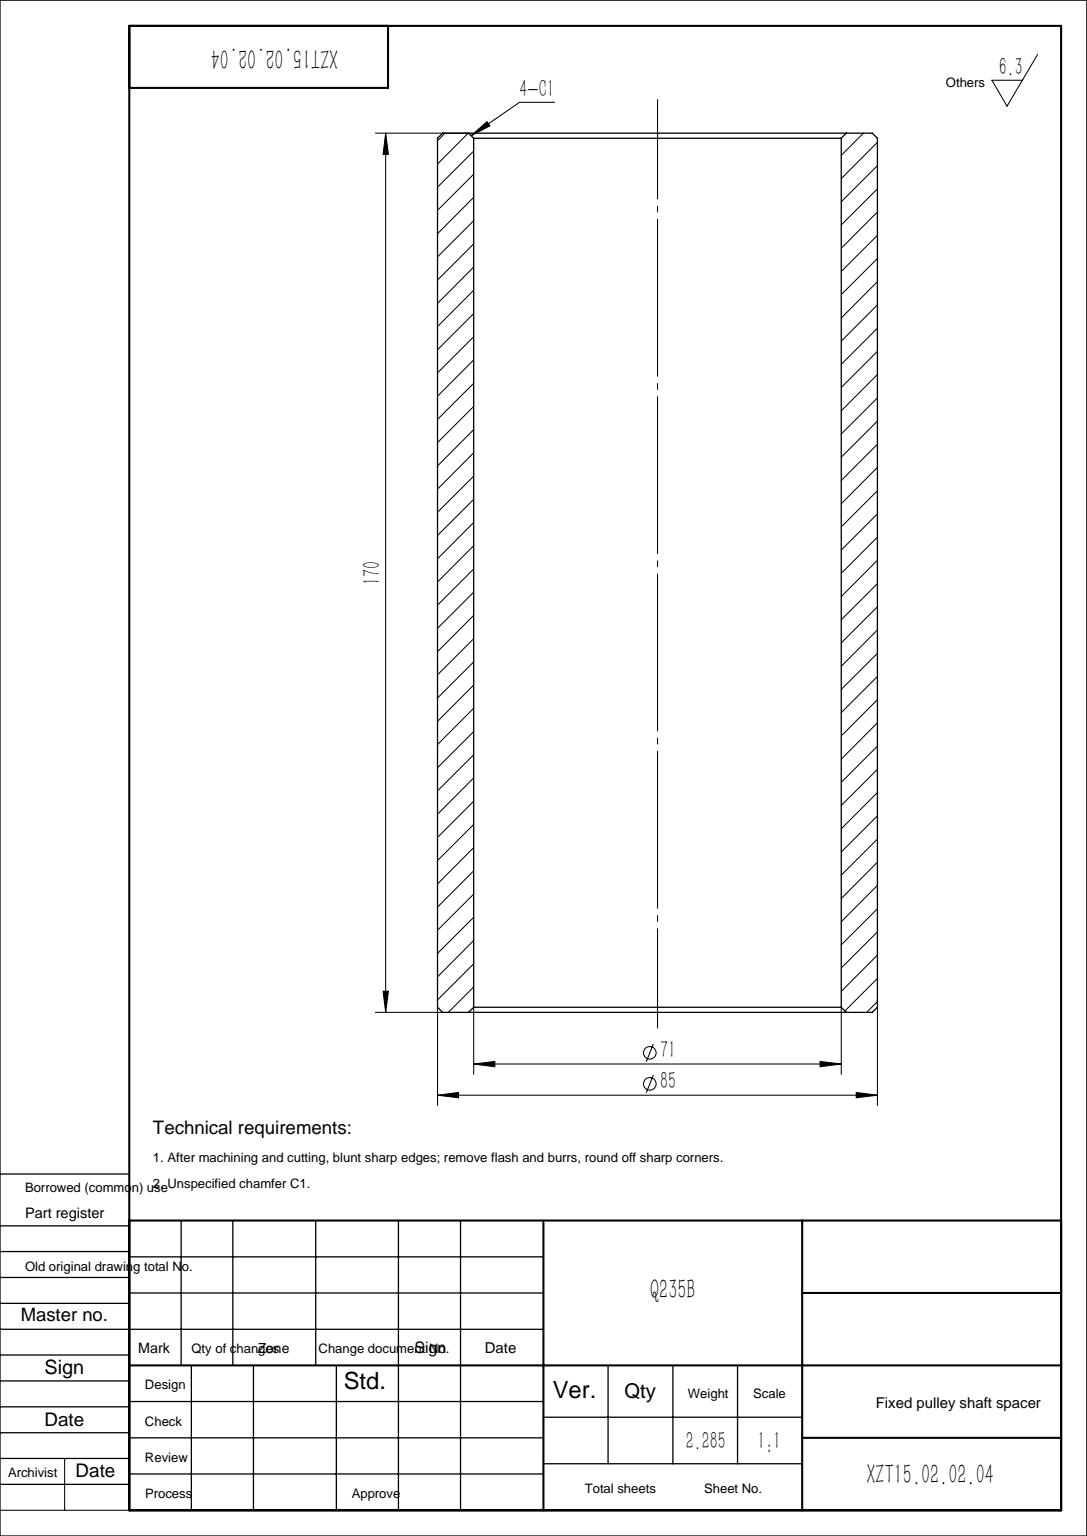
from build123d import *

# Parameters (mm, degrees)
SKETCH1_R           = 42.5
SKETCH1_R_2         = 35.5
BOSS_EXTRUDE1_DEPTH = 170
CHAMFER2_SIZE       = 1


with BuildPart() as part:
    # Sketch1 → Boss-Extrude1 (new body)
    with BuildSketch(Plane(origin=(0, 0, 0), x_dir=(1, 0, 0), z_dir=(0, 1, 0))):
        with Locations(Location((0, 0, 0), (0, 0, 270))):
            Circle(SKETCH1_R)
        with Locations(Location((0, 0, 0), (0, 0, 270))):
            Circle(SKETCH1_R_2, mode=Mode.SUBTRACT)
    extrude(amount=BOSS_EXTRUDE1_DEPTH)

    # Chamfer2
    chamfer2_edges = [part.edges().sort_by_distance(p)[0] for p in [
        (0, 0, -42.5),
        (0, 170, -42.5),
        (0, 0, -35.5),
        (0, 170, -35.5),
    ]]
    chamfer(chamfer2_edges, length=CHAMFER2_SIZE)


solid = part.part
